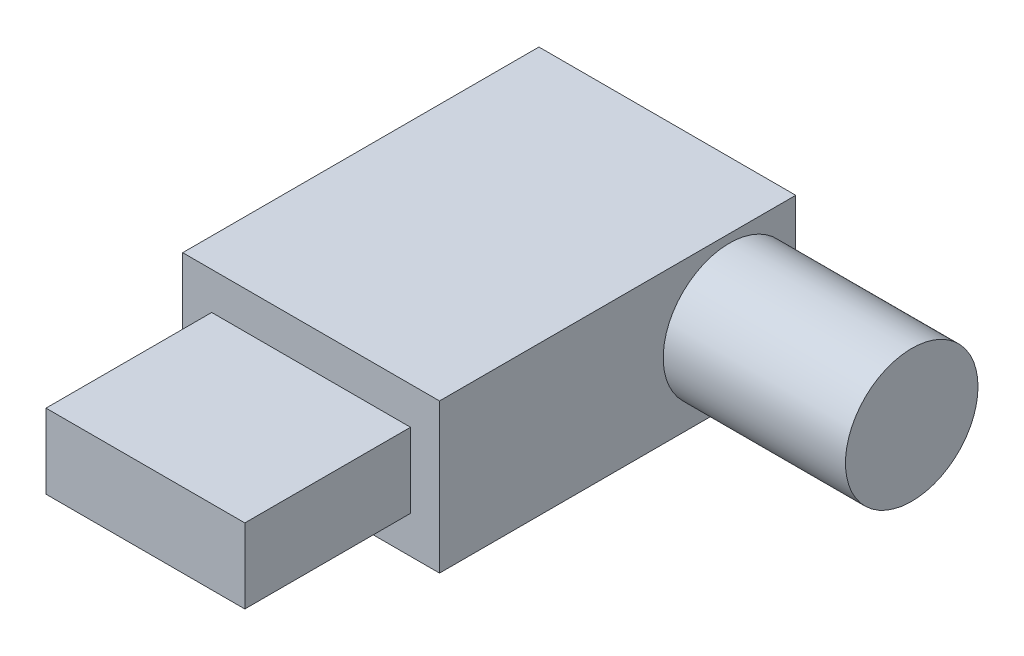
SolidWorks part; units mm, degrees
ref_plane "前视基准面" through (0, 0, 0) normal (0, 0, 1) x (1, 0, 0)
ref_plane "上视基准面" through (0, 0, 0) normal (0, 1, 0) x (1, 0, 0)
ref_plane "右视基准面" through (0, 0, 0) normal (1, 0, 0) x (0, 0, -1)
sketch "草图1" plane through (0, 0, 0) normal (0, 0, 1) x (1, 0, 0)
  line L1 (-7.75, -4.5) -> (7.75, -4.5)
  line L2 (-7.75, -4.5) -> (-7.75, 4.5)
  line L3 (-7.75, 4.5) -> (7.75, 4.5)
  line L4 (7.75, -4.5) -> (7.75, 4.5)
  line L5 (-7.75, -4.5) -> (7.75, 4.5) construction
  line L6 (-7.75, 4.5) -> (7.75, -4.5) construction
  point P0 (0, 0)
  dimension "D1" = 15.5
  dimension "D2" = 9
extrude "凸台-拉伸1" add sketch "草图1" against normal blind 21.5
sketch "草图2" plane through (7.75, 0, 0) normal (1, 0, 0) x (0, 0, -1)
  line L0 (0, 0) -> (21.5, 0) construction
  line L1 (21.5, -4.5) -> (21.5, 4.5) construction
  circle A0 centre (17.5, 0) radius 4
  dimension "D1" = 8
  dimension "D2" = 4
extrude "凸台-拉伸2" add sketch "草图2" along normal blind 11
sketch "草图3" plane through (0, 0, 0) normal (0, 0, 1) x (1, 0, 0)
  line L1 (-6, -2.25) -> (6, -2.25)
  line L2 (-6, -2.25) -> (-6, 2.25)
  line L3 (-6, 2.25) -> (6, 2.25)
  line L4 (6, -2.25) -> (6, 2.25)
  line L5 (-6, -2.25) -> (6, 2.25) construction
  line L6 (-6, 2.25) -> (6, -2.25) construction
  point P0 (0, 0)
  dimension "D1" = 12
  dimension "D2" = 4.5
extrude "凸台-拉伸3" add sketch "草图3" along normal blind 10
